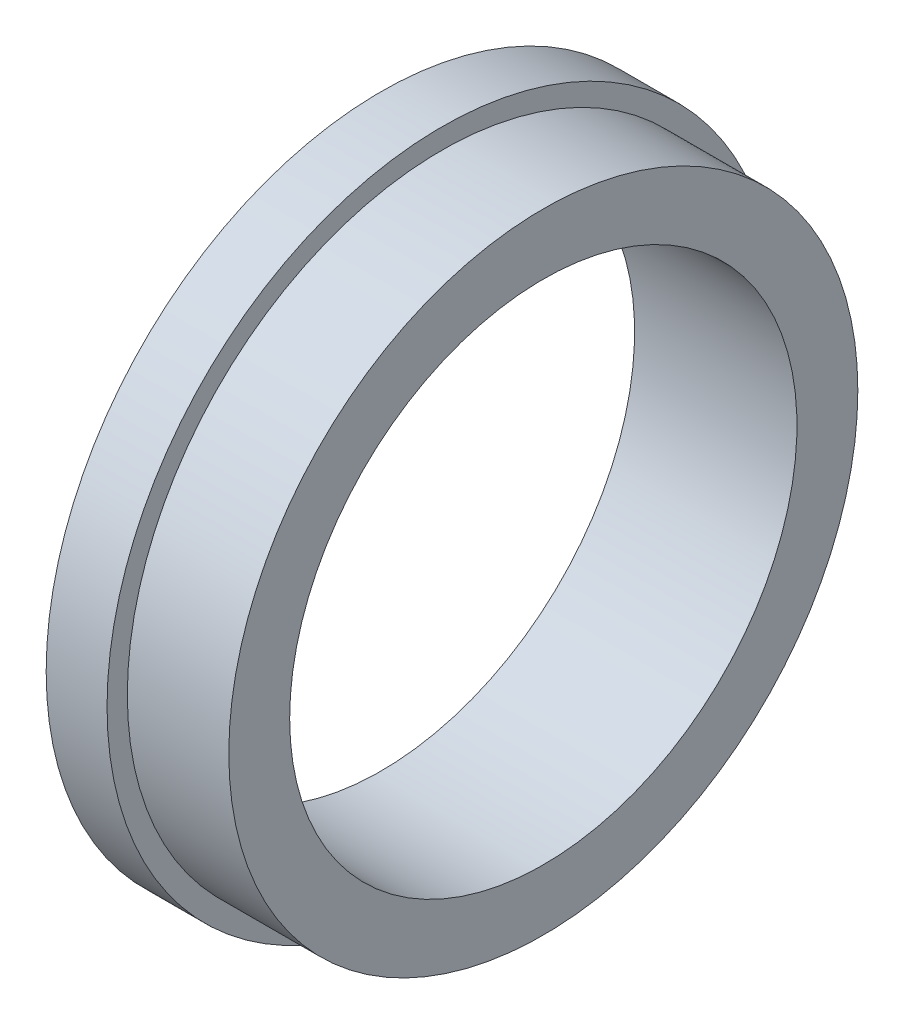
from build123d import *


with BuildPart() as part:
    # Sketch1 → Revolve1 (revolve)
    with BuildSketch(Plane.XY, mode=Mode.PRIVATE) as revolve1_sk:
        Polygon((0, 25), (16, 25), (16, 31), (6, 31), (6, 33), (0, 33), align=None)
    revolve(revolve1_sk.sketch.rotate(Axis((0, 0, 0), (1, 0, 0)), 90), axis=Axis((0, 0, 0), (1, 0, 0)))


solid = part.part
